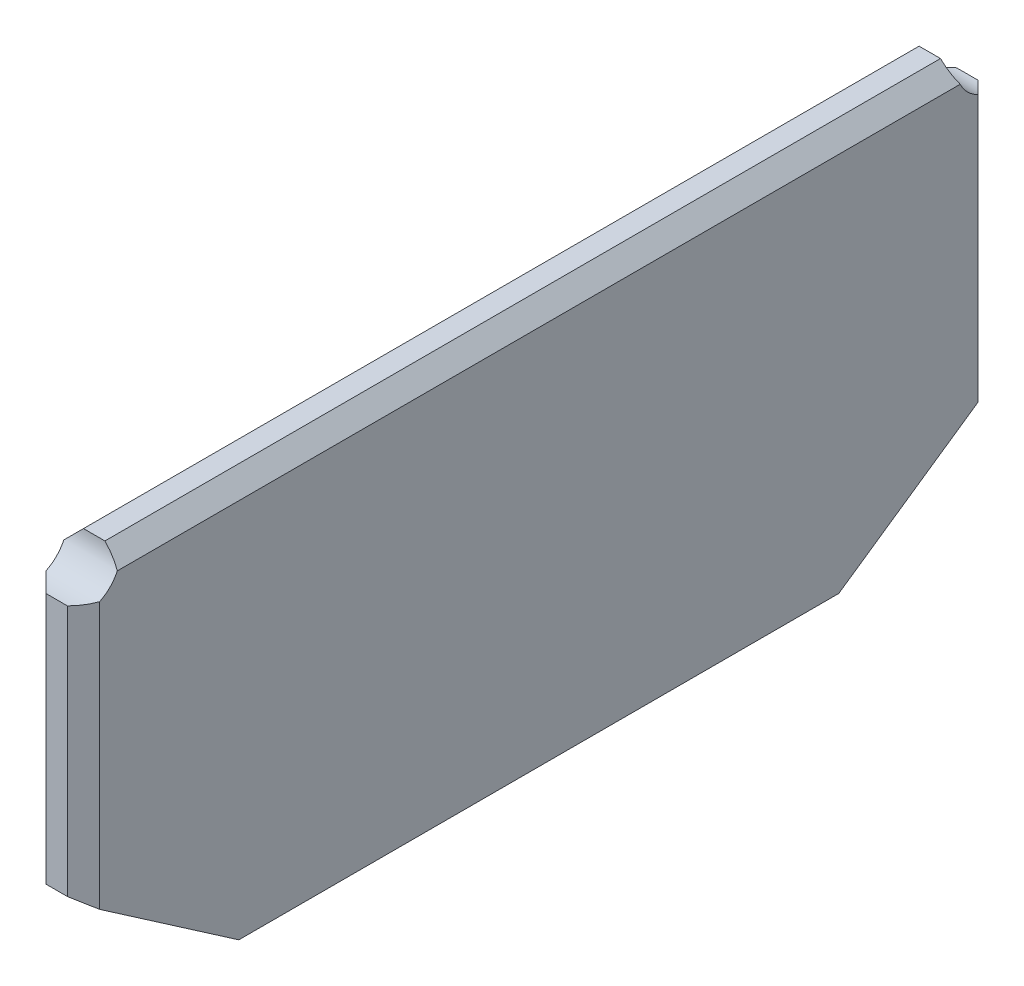
from build123d import *

# Parameters (mm, degrees)
BOSS_EXTRUDE1_DEPTH = 25
CHAMFER1_SIZE       = 15


with BuildPart() as part:
    # Sketch1 → Boss-Extrude1 (new, symmetric)
    with BuildSketch(Plane(origin=(0, 0, 0), x_dir=(0, 0, -1), z_dir=(1, 0, 0))):
        with BuildLine():
            Line((-390, 370), (390, 370))
            ThreePointArc((390, 370), (400.251262658, 345.251262658), (425, 335))
            Line((425, 335), (425, 100))
            Line((425, 100), (280, 0))
            Line((280, 0), (-280, 0))
            Line((-280, 0), (-425, 100))
            Line((-425, 100), (-425, 335))
            ThreePointArc((-425, 335), (-400.251262658, 345.251262658), (-390, 370))
        make_face()
    extrude(amount=BOSS_EXTRUDE1_DEPTH, both=True)

    # Chamfer1
    chamfer1_edges = [part.edges().sort_by_distance(p)[0] for p in [
        (-25, 370, 0),
        (25, 217.5, 425),
        (25, 217.5, -425),
        (25, 370, 0),
        (-25, 217.5, -425),
        (-25, 217.5, 425),
    ]]
    chamfer(chamfer1_edges, length=CHAMFER1_SIZE)


solid = part.part
